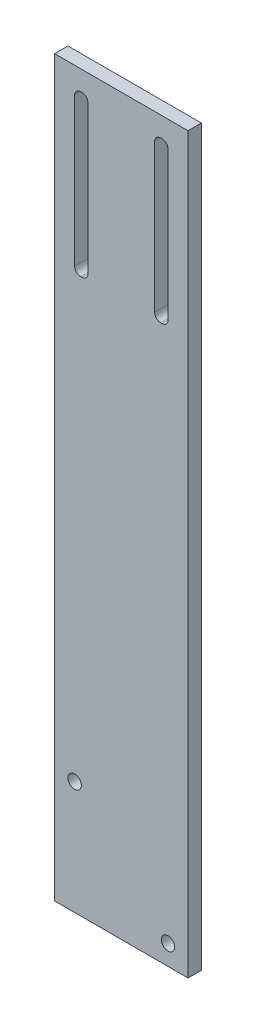
SolidWorks part; units mm, degrees
material "PVC Rigid"
ref_plane "Front Plane" through (0, 0, 0) normal (0, 0, 1) x (1, 0, 0)
ref_plane "Top Plane" through (0, 0, 0) normal (0, 1, 0) x (1, 0, 0)
ref_plane "Right Plane" through (0, 0, 0) normal (1, 0, 0) x (0, 0, -1)
sketch "Sketch1" plane through (0, 0, 0) normal (0, 0, 1) x (1, 0, 0)
  line L1 (50, -275) -> (-50, -275)
  line L2 (50, -275) -> (50, 275)
  line L3 (50, 275) -> (-50, 275)
  line L4 (-50, -275) -> (-50, 275)
  line L5 (50, -275) -> (-50, 275) construction
  line L6 (50, 275) -> (-50, -275) construction
  point P0 (0, 0)
  dimension "D1" = 100
  dimension "D2" = 550
extrude "Boss-Extrude1" add sketch "Sketch1" along normal blind 10
sketch "Sketch2" plane through (0, 0, 10) normal (0, 0, 1) x (1, 0, 0)
  line L0 (50, -275) -> (-50, -175) construction
  line L1 (-50, 275) -> (-50, -275) construction
  line L2 (-50, -275) -> (50, -275) construction
  line L3 (50, -275) -> (50, 275) construction
  circle A0 centre (-35, -190) radius 5
  circle A1 centre (35, -260) radius 5
  dimension "D4" = 10
  dimension "D5" = 10
  dimension "D1" = 45
  dimension "D2" = 15
  dimension "D3" = 15
extrude "Cut-Extrude1" cut sketch "Sketch2" against normal blind 10
sketch "Sketch3" plane through (0, 0, 10) normal (0, 0, 1) x (1, 0, 0)
  line L0 (0, 253.6663) -> (0, 286.3594) construction
  line L1 (-25, 275) -> (-25, 223.2436) construction
  line L2 (50, 275) -> (-50, 275) construction
  line L3 (25, 275) -> (25, 211.3422) construction
  line L4 (-50, 275) -> (-50, -275) construction
  line L5 (-29.5, 140.0997) -> (-30.5, 140.0997)
  line L6 (-25, 144.5997) -> (-25, 255.5997)
  line L7 (-29.5, 260.0997) -> (-30.5, 260.0997)
  line L8 (-35, 144.5997) -> (-35, 255.5997)
  line L9 (-25, 140.0997) -> (-35, 260.0997) construction
  line L10 (-25, 260.0997) -> (-35, 140.0997) construction
  line L11 (30.5, 140.0997) -> (29.5, 140.0997)
  line L12 (35, 144.5997) -> (35, 255.5997)
  line L13 (30.5, 260.0997) -> (29.5, 260.0997)
  line L14 (25, 144.5997) -> (25, 255.5997)
  line L15 (35, 140.0997) -> (25, 260.0997) construction
  line L16 (35, 260.0997) -> (25, 140.0997) construction
  line L17 (50, -275) -> (50, 275) construction
  arc A0 (29.5, 260.0997) -> (25, 255.5997) centre (29.5, 255.5997) ccw
  arc A1 (35, 255.5997) -> (30.5, 260.0997) centre (30.5, 255.5997) ccw
  arc A2 (30.5, 140.0997) -> (35, 144.5997) centre (30.5, 144.5997) ccw
  arc A3 (29.5, 140.0997) -> (25, 144.5997) centre (29.5, 144.5997) cw
  arc A4 (-30.5, 140.0997) -> (-35, 144.5997) centre (-30.5, 144.5997) cw
  arc A5 (-29.5, 140.0997) -> (-25, 144.5997) centre (-29.5, 144.5997) ccw
  arc A6 (-25, 255.5997) -> (-29.5, 260.0997) centre (-29.5, 255.5997) ccw
  arc A7 (-30.5, 260.0997) -> (-35, 255.5997) centre (-30.5, 255.5997) ccw
  point P9 (-30, 200.0997)
  point P14 (30, 200.0997)
  dimension "D7" = 4.5
  dimension "D1" = 15
  dimension "D2" = 15
  dimension "D3" = 10
  dimension "D4" = 10
  dimension "D5" = 120
  dimension "D6" = 120
extrude "Cut-Extrude2" cut sketch "Sketch3" against normal blind 10
